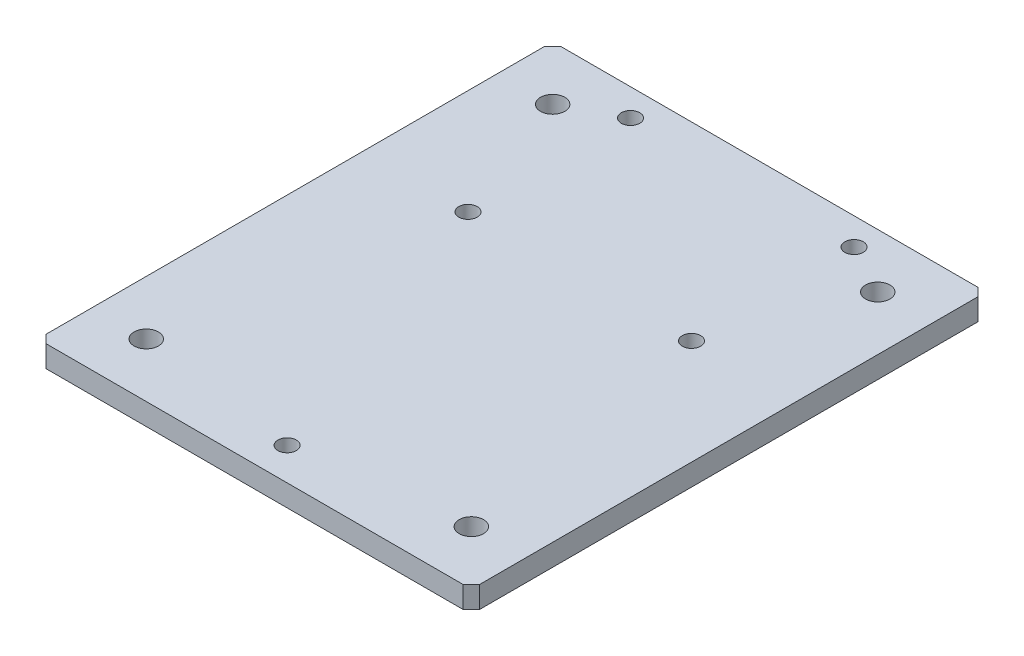
SolidWorks part; units mm, degrees
material "A6061"
ref_plane "前基準面" through (0, 0, 0) normal (0, 0, 1) x (1, 0, 0)
ref_plane "上基準面" through (0, 0, 0) normal (0, 1, 0) x (1, 0, 0)
ref_plane "右基準面" through (0, 0, 0) normal (1, 0, 0) x (0, 0, -1)
sketch "草图1" plane through (0, 0, 0) normal (0, 1, 0) x (1, 0, 0)
  line L1 (-80, -95) -> (80, -95)
  line L2 (-80, -95) -> (-80, 95)
  line L3 (-80, 95) -> (80, 95)
  line L4 (80, -95) -> (80, 95)
  line L5 (-80, -95) -> (80, 95) construction
  line L6 (-80, 95) -> (80, -95) construction
  point P0 (0, 0)
  dimension "D1" = 160
  dimension "D2" = 190
extrude "凸台-拉伸1" add sketch "草图1" along normal mid plane 8
chamfer "倒角1" distance 3 angle 45 4 edges at (80, 0, -95) (80, 0, 95) (-80, 0, -95) (-80, 0, 95)
hole_wizard "Ø9.0 (9) 直径孔1" positions "草图2" profile "草图3" hole size "Ø9.0" standard "GB" end condition through all
sketch "草图2" plane through (0, -4, 0) normal (0, -1, 0) x (-1, 0, 0)
  line L0 (-91.9584, 0) -> (0, 0) construction
  line L1 (0, 0) -> (0, -82.4209) construction
  line L3 (77, -95) -> (-77, -95) construction
  line L4 (-80, -92) -> (-80, 92) construction
  point P0 (-60, -75)
  point P10 (60, -75)
  point P11 (60, 75)
  point P12 (-60, 75)
  dimension "D1" = 20
  dimension "D2" = 20
sketch "草图3" plane through (60, -4, 75) normal (1, 0, 0) x (0, 0, -1)
  line L0 (0, 0) -> (0, 8)
  line L1 (0, 8) -> (4.5, 8)
  line L2 (4.5, 8) -> (4.5, 0)
  line L5 (4.5, 0) -> (0, 0)
  line L11 (0, -6.35) -> (0, 107.95) construction
  dimension "通孔孔直径" = 9
  dimension "通孔孔深度" = 8
hole_wizard "M8 螺纹孔2" positions "草图4" profile "草图5" tap size "M8" standard "GB" end condition through all
sketch "草图4" plane through (0, -4, 0) normal (0, -1, 0) x (-1, 0, 0)
  line L0 (-106.5155, 55) -> (0, 55) construction
  line L1 (0, 55) -> (0, -83.9342) construction
  line L2 (-77, 95) -> (77, 95) construction
  point P0 (-41.25, 25)
  point P11 (-41.25, 85)
  point P12 (41.25, 85)
  point P13 (41.25, 25)
  dimension "D1" = 82.5
  dimension "D2" = 60
  dimension "D3" = 10
sketch "草图5" plane through (41.25, -4, -25) normal (1, 0, 0) x (0, 0, -1)
  line L0 (0, 0) -> (0, 8)
  line L1 (0, 8) -> (3.4, 8)
  line L2 (3.4, 8) -> (3.4, 0)
  line L5 (3.4, 0) -> (0, 0)
  line L11 (0, -6.35) -> (0, 107.95) construction
  dimension "通孔螺纹孔钻头直径" = 6.8
  dimension "通孔螺纹孔钻头深度" = 8
cosmetic thread "孔螺蚊线1" parameters "D2"=8
cosmetic thread "孔螺蚊线2" parameters "D2"=8
cosmetic thread "孔螺蚊线3" parameters "D2"=8
cosmetic thread "孔螺蚊线4" parameters "D2"=8
hole_wizard "M8 螺纹孔1" positions "草图6" profile "草图7" tap size "M8" standard "GB" end condition through all
sketch "草图6" plane through (0, -4, 0) normal (0, -1, 0) x (-1, 0, 0)
  line L0 (0, -123.6763) -> (0, 0) construction
  line L2 (77, -95) -> (-77, -95) construction
  point P0 (0, -83)
  dimension "D1" = 12
sketch "草图7" plane through (0, -4, 83) normal (1, 0, 0) x (0, 0, -1)
  line L0 (0, 0) -> (0, 8)
  line L1 (0, 8) -> (3.4, 8)
  line L2 (3.4, 8) -> (3.4, 0)
  line L5 (3.4, 0) -> (0, 0)
  line L11 (0, -6.35) -> (0, 107.95) construction
  dimension "通孔螺纹孔钻头直径" = 6.8
  dimension "通孔螺纹孔钻头深度" = 8
cosmetic thread "孔螺蚊线6" parameters "D2"=8
